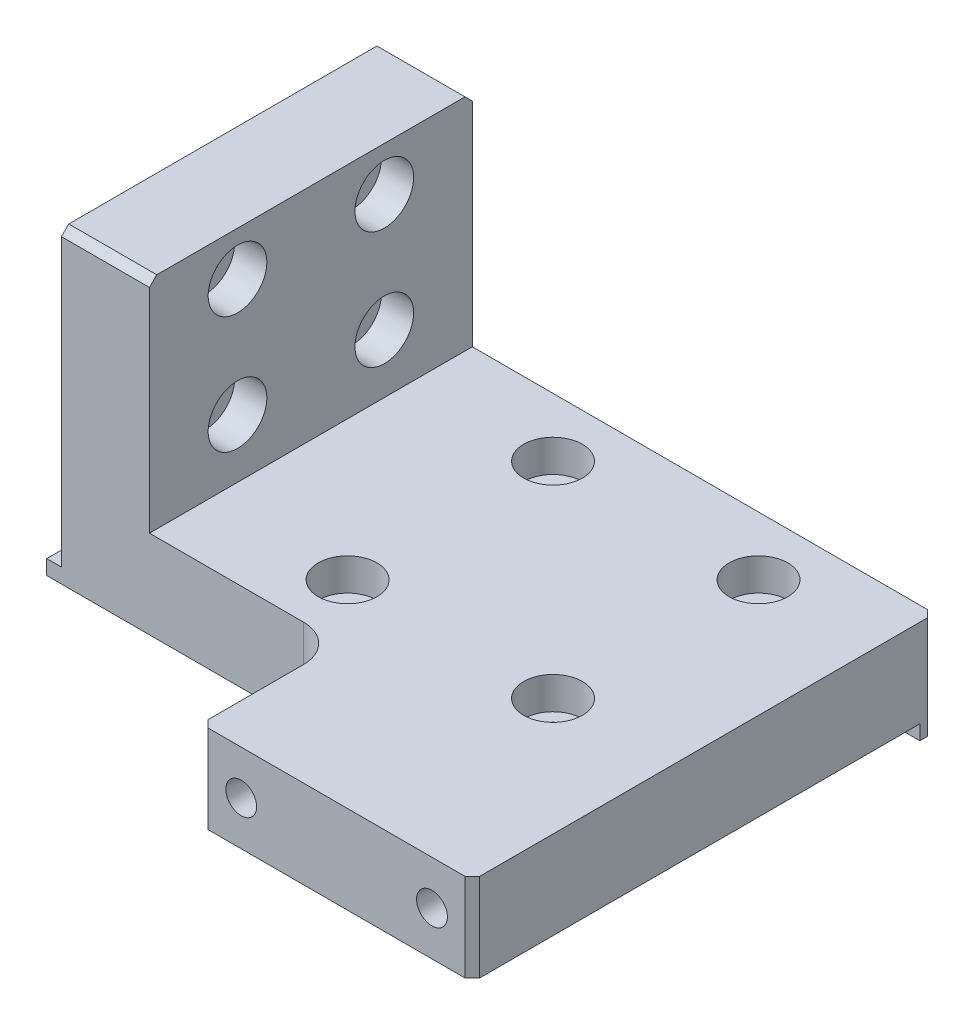
from build123d import *

# Parameters (mm, degrees)
SKETCH1_W                                           = 75
SKETCH1_H                                           = 12
BOSS_EXTRUDE1_DEPTH                                 = 73
SKETCH2_W                                           = 75
SKETCH2_H                                           = 2
BOSS_EXTRUDE2_DEPTH                                 = 2
SKETCH3_W                                           = 75
SKETCH3_H                                           = 10
BOSS_EXTRUDE3_DEPTH                                 = 15
SKETCH4_W                                           = 12
SKETCH4_H                                           = 63
BOSS_EXTRUDE4_DEPTH                                 = 30
SKETCH5_W                                           = 63
SKETCH5_H                                           = 2
BOSS_EXTRUDE5_DEPTH                                 = 2
SKETCH7_W                                           = 40
SKETCH7_H                                           = 42
CUT_EXTRUDE2_DEPTH                                  = 29
M5_TAPPED_HOLE1_D                                   = 4.2
M5_TAPPED_HOLE1_DEPTH                               = 12.4
M5_TAPPED_HOLE1_TIP                                 = 1.2618073
CBORE_FOR_M4_HEX_SOCKET_HEAD_CAP_SCREW1_D           = 4.5
CBORE_FOR_M4_HEX_SOCKET_HEAD_CAP_SCREW1_CBORE_D     = 8
CBORE_FOR_M4_HEX_SOCKET_HEAD_CAP_SCREW1_CBORE_DEPTH = 4.4
SKETCH12_W                                          = 37
SKETCH12_H                                          = 10
CUT_EXTRUDE3_DEPTH                                  = 88.92184029
M5_TAPPED_HOLE2_D                                   = 4.2
M5_TAPPED_HOLE2_DEPTH                               = 12.4
M5_TAPPED_HOLE2_TIP                                 = 1.2618073
FILLET1_R                                           = 5
CBORE_FOR_M4_HEX_SOCKET_HEAD_CAP_SCREW2_D           = 4.5
CBORE_FOR_M4_HEX_SOCKET_HEAD_CAP_SCREW2_CBORE_D     = 8
CBORE_FOR_M4_HEX_SOCKET_HEAD_CAP_SCREW2_CBORE_DEPTH = 4.4
CHAMFER1_SIZE                                       = 1


with BuildPart() as part:
    # Sketch1 → Boss-Extrude1 (new body)
    with BuildSketch(Plane.XY):
        Rectangle(SKETCH1_W, SKETCH1_H)
    extrude(amount=BOSS_EXTRUDE1_DEPTH)

    # Sketch2 → Boss-Extrude2 (add)
    with BuildSketch(Plane.XZ.offset(6)):
        with Locations((0, 1)):
            Rectangle(SKETCH2_W, SKETCH2_H)
    extrude(amount=BOSS_EXTRUDE2_DEPTH)

    # Sketch3 → Boss-Extrude3 (add)
    with BuildSketch(Plane(origin=(0, 6, 0), x_dir=(1, 0, 0), z_dir=(0, 1, 0))):
        with Locations((0, -68)):
            Rectangle(SKETCH3_W, SKETCH3_H)
    extrude(amount=BOSS_EXTRUDE3_DEPTH)

    # Sketch4 → Boss-Extrude4 (add)
    with BuildSketch(Plane(origin=(0, 6, 0), x_dir=(1, 0, 0), z_dir=(0, 1, 0))):
        with Locations((-31.5, -31.5)):
            Rectangle(SKETCH4_W, SKETCH4_H)
    extrude(amount=BOSS_EXTRUDE4_DEPTH)

    # Sketch5 → Boss-Extrude5 (add)
    with BuildSketch(Plane.ZY.offset(37.5)):
        with Locations((31.5, -5)):
            Rectangle(SKETCH5_W, SKETCH5_H)
    extrude(amount=BOSS_EXTRUDE5_DEPTH)

    # Sketch7 → Cut-Extrude2 (cut)
    with BuildSketch(Plane.XY.offset(73)):
        with Locations((-19.5, 15)):
            Rectangle(SKETCH7_W, SKETCH7_H)
    extrude(amount=-CUT_EXTRUDE2_DEPTH, mode=Mode.SUBTRACT)

    # M5 Tapped Hole1
    with Locations(Plane.XY.offset(73)):
        with Locations((19, 10)):
            Hole(M5_TAPPED_HOLE1_D / 2, depth=M5_TAPPED_HOLE1_DEPTH)
            with Locations((0, 0, -(M5_TAPPED_HOLE1_DEPTH + M5_TAPPED_HOLE1_TIP / 2))):  # 118° drill point
                Cone(0, M5_TAPPED_HOLE1_D / 2, M5_TAPPED_HOLE1_TIP, mode=Mode.SUBTRACT)

    # CBORE for M4 Hex Socket Head Cap Screw1 (through all)
    with Locations(Plane(origin=(-25.5, 0, 0), x_dir=(0, 0, -1), z_dir=(1, 0, 0))):
        with Locations((-32, 30), (-32, 14), (-12, 14), (-12, 30)):
            CounterBoreHole(CBORE_FOR_M4_HEX_SOCKET_HEAD_CAP_SCREW1_D / 2, CBORE_FOR_M4_HEX_SOCKET_HEAD_CAP_SCREW1_CBORE_D / 2, CBORE_FOR_M4_HEX_SOCKET_HEAD_CAP_SCREW1_CBORE_DEPTH)

    # Sketch12 → Cut-Extrude3 (cut, through all)
    with BuildSketch(Plane(origin=(0, 21, 0), x_dir=(1, 0, 0), z_dir=(0, 1, 0))):
        with Locations((19, -68)):
            Rectangle(SKETCH12_W, SKETCH12_H)
    extrude(amount=-CUT_EXTRUDE3_DEPTH, mode=Mode.SUBTRACT)

    # M5 Tapped Hole2
    with Locations(Plane.XY.offset(63)):
        with Locations((32, 0), (6, 0)):
            Hole(M5_TAPPED_HOLE2_D / 2, depth=M5_TAPPED_HOLE2_DEPTH)
            with Locations((0, 0, -(M5_TAPPED_HOLE2_DEPTH + M5_TAPPED_HOLE2_TIP / 2))):  # 118° drill point
                Cone(0, M5_TAPPED_HOLE2_D / 2, M5_TAPPED_HOLE2_TIP, mode=Mode.SUBTRACT)

    # Fillet1
    fillet1_edges = [part.edges().sort_by_distance(p)[0] for p in [
        (0.5, 0, 44),
    ]]
    fillet(fillet1_edges, radius=FILLET1_R)

    # CBORE for M4 Hex Socket Head Cap Screw2 (through all)
    with Locations(Plane(origin=(0, 6, 0), x_dir=(1, 0, 0), z_dir=(0, 1, 0))):
        with Locations((-6.5, -8), (21.5, -8), (-6.5, -36), (21.5, -36)):
            CounterBoreHole(CBORE_FOR_M4_HEX_SOCKET_HEAD_CAP_SCREW2_D / 2, CBORE_FOR_M4_HEX_SOCKET_HEAD_CAP_SCREW2_CBORE_D / 2, CBORE_FOR_M4_HEX_SOCKET_HEAD_CAP_SCREW2_CBORE_DEPTH)

    # Chamfer1
    chamfer1_edges = [part.edges().sort_by_distance(p)[0] for p in [
        (0.5, 0, 63),
        (37.5, 0, 63),
        (37.5, -1, 0),
        (-31.5, 36, 0),
        (-31.5, 36, 44),
    ]]
    chamfer(chamfer1_edges, length=CHAMFER1_SIZE)


solid = part.part
